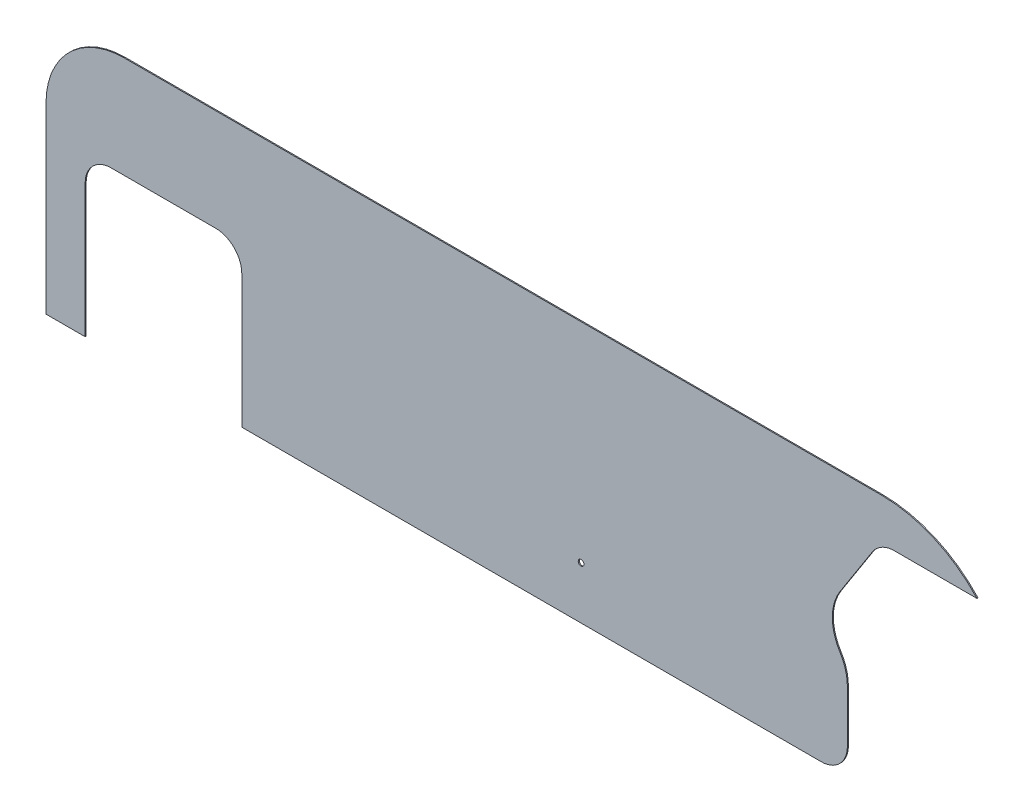
SolidWorks part; units mm, degrees
material "普通碳钢"
ref_plane "Front Plane" through (0, 0, 0) normal (0, 0, 1) x (1, 0, 0)
ref_plane "Top Plane" through (0, 0, 0) normal (0, 1, 0) x (1, 0, 0)
ref_plane "Right Plane" through (0, 0, 0) normal (1, 0, 0) x (0, 0, -1)
sketch "Sketch1" plane through (0, 0, 0) normal (0, 0, 1) x (1, 0, 0)
  line L0 (186.2359, 172.72) -> (25.4, 172.72)
  line L1 (-17.3586, 149.3489) -> (-80.1724, 51.4291)
  line L2 (-66.04, -101.3696) -> (-66.04, -203.2)
  line L3 (0, 254) -> (-1473.2, 254)
  line L4 (-116.84, -254) -> (-1244.6, -254)
  line L5 (-1625.6, 101.6) -> (-1625.6, -254)
  line L6 (-1549.4, -254) -> (-1549.4, 5.08)
  line L7 (-1498.6, 55.88) -> (-1295.4, 55.88)
  line L8 (-1244.6, 5.08) -> (-1244.6, -254)
  line L9 (-1549.4, -254) -> (-1625.6, -254)
  arc A0 (-80.1724, 51.4291) -> (-80.645, -50.6848) centre (0, 0) ccw
  arc A1 (186.2359, 172.72) -> (0, 254) centre (0, 0) ccw
  arc A2 (25.4, 172.72) -> (-17.3586, 149.3489) centre (25.4, 121.92) ccw
  arc A3 (-1473.2, 254) -> (-1625.6, 101.6) centre (-1473.2, 101.6) ccw
  arc A4 (-66.04, -203.2) -> (-116.84, -254) centre (-116.84, -203.2) cw
  arc A5 (-66.04, -101.3696) -> (-80.645, -50.6848) centre (-161.29, -101.3696) ccw
  arc A6 (-1295.4, 55.88) -> (-1244.6, 5.08) centre (-1295.4, 5.08) cw
  arc A7 (-1549.4, 5.08) -> (-1498.6, 55.88) centre (-1498.6, 5.08) cw
  circle A8 centre (-584.2, -152.4) radius 5.588
  point P24 (-1244.6, 55.88)
  point P27 (-1549.4, 55.88)
  dimension "D1" = 190.5
  dimension "D2" = 508
  dimension "D4" = 25.4
  dimension "D5" = 101.6
  dimension "D6" = 152.4
  dimension "D9" = 50.8
  dimension "D10" = 95.25
  dimension "D14" = 50.8
  dimension "D15" = 518.16
  dimension "D17" = 11.176
  dimension "D3" = 172.72
  dimension "D7" = 1625.6
  dimension "D8" = 1559.56
  dimension "D11" = 309.88
  dimension "D12" = 304.8
  dimension "D13" = 76.2
  dimension "D16" = 152.4
extrude "Boss-Extrude1" add sketch "Sketch1" along normal mid plane 2
